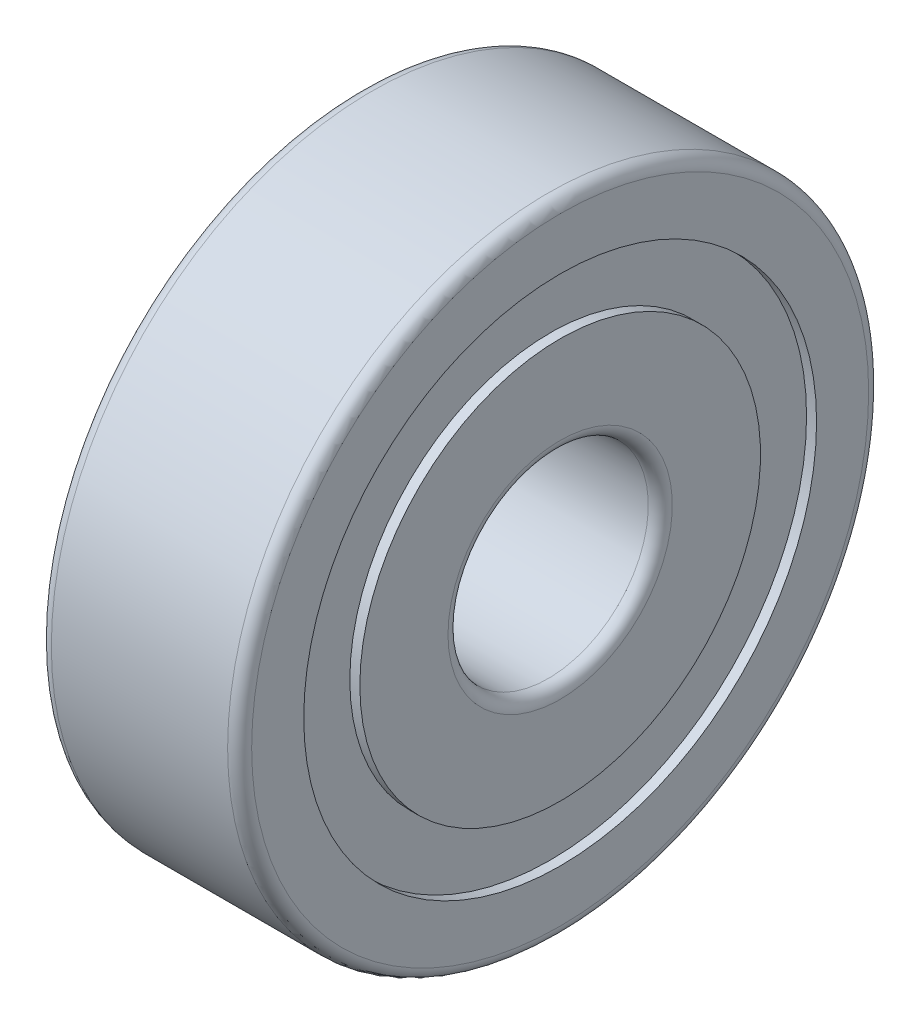
SolidWorks part; units mm, degrees
ref_plane "前视基准面" through (0, 0, 0) normal (0, 0, 1) x (1, 0, 0)
ref_plane "上视基准面" through (0, 0, 0) normal (0, 1, 0) x (1, 0, 0)
ref_plane "右视基准面" through (0, 0, 0) normal (1, 0, 0) x (0, 0, -1)
sketch "草图1" plane through (0, 0, 0) normal (0, 0, 1) x (1, 0, 0)
  line L0 (-2.5, 7.7) -> (-2.5, 6.4)
  line L1 (-2.5, 6.4) -> (-2.25, 6.4)
  line L2 (-2.25, 6.4) -> (-2.25, 5)
  line L3 (-2.25, 5) -> (-2.5, 5)
  line L4 (-2.5, 5) -> (-2.5, 2.8)
  line L5 (-2.2, 2.5) -> (2.2, 2.5)
  line L6 (2.5, 2.8) -> (2.5, 5)
  line L7 (2.5, 5) -> (2.25, 5)
  line L8 (2.25, 5) -> (2.25, 6.4)
  line L9 (2.25, 6.4) -> (2.5, 6.4)
  line L10 (2.5, 6.4) -> (2.5, 7.7)
  line L11 (2.2, 8) -> (-2.2, 8)
  line L12 (2.5, 0) -> (-2.5, 0) construction
  arc A0 (-2.5, 2.8) -> (-2.2, 2.5) centre (-2.2, 2.8) ccw
  arc A1 (2.2, 2.5) -> (2.5, 2.8) centre (2.2, 2.8) ccw
  arc A2 (2.5, 7.7) -> (2.2, 8) centre (2.2, 7.7) ccw
  arc A3 (-2.2, 8) -> (-2.5, 7.7) centre (-2.2, 7.7) ccw
revolve "旋转1" add sketch "草图1" angle 360 about L12
